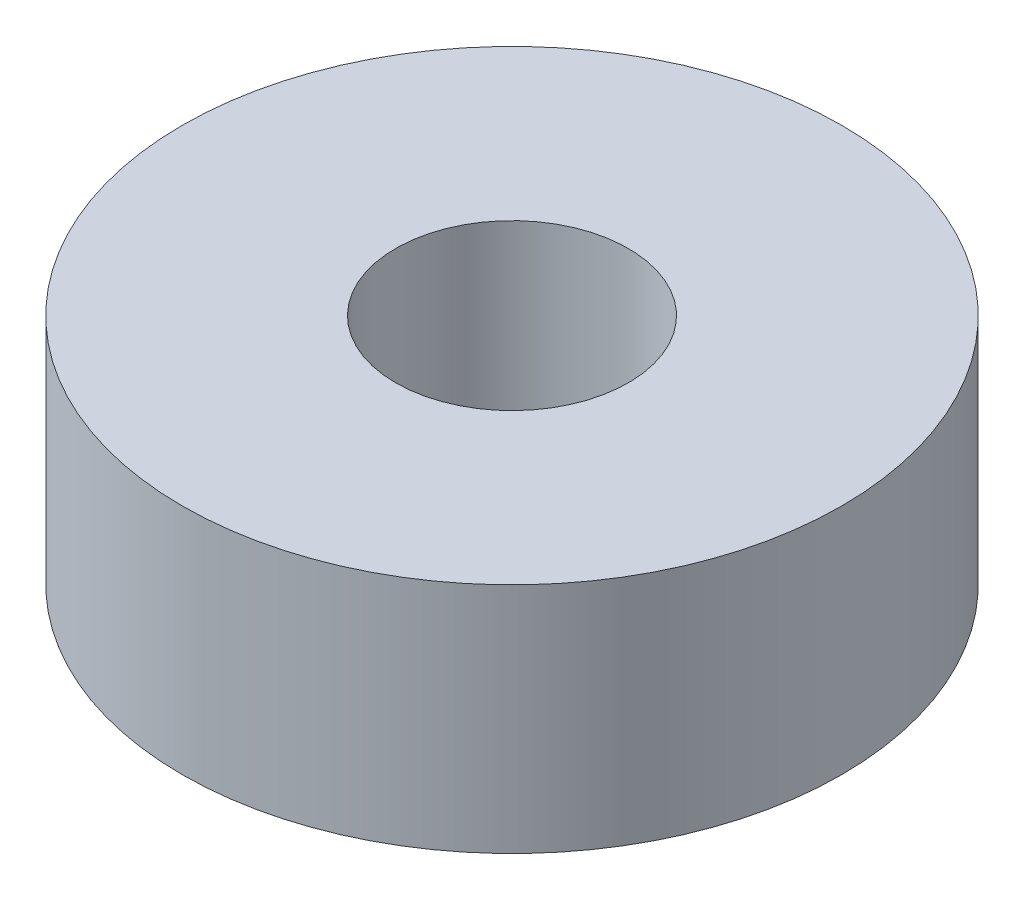
from build123d import *

# Parameters (mm, degrees)
SKETCH1_R           = 8.5
SKETCH1_R_2         = 3
BOSS_EXTRUDE1_DEPTH = 6


with BuildPart() as part:
    # Sketch1 → Boss-Extrude1 (new body)
    with BuildSketch(Plane(origin=(0, 0, 0), x_dir=(1, 0, 0), z_dir=(0, 1, 0))):
        with Locations(Location((0, 0, 0), (0, 0, 270))):
            Circle(SKETCH1_R)
        with Locations(Location((0, 0, 0), (0, 0, 270))):
            Circle(SKETCH1_R_2, mode=Mode.SUBTRACT)
    extrude(amount=BOSS_EXTRUDE1_DEPTH)


solid = part.part
